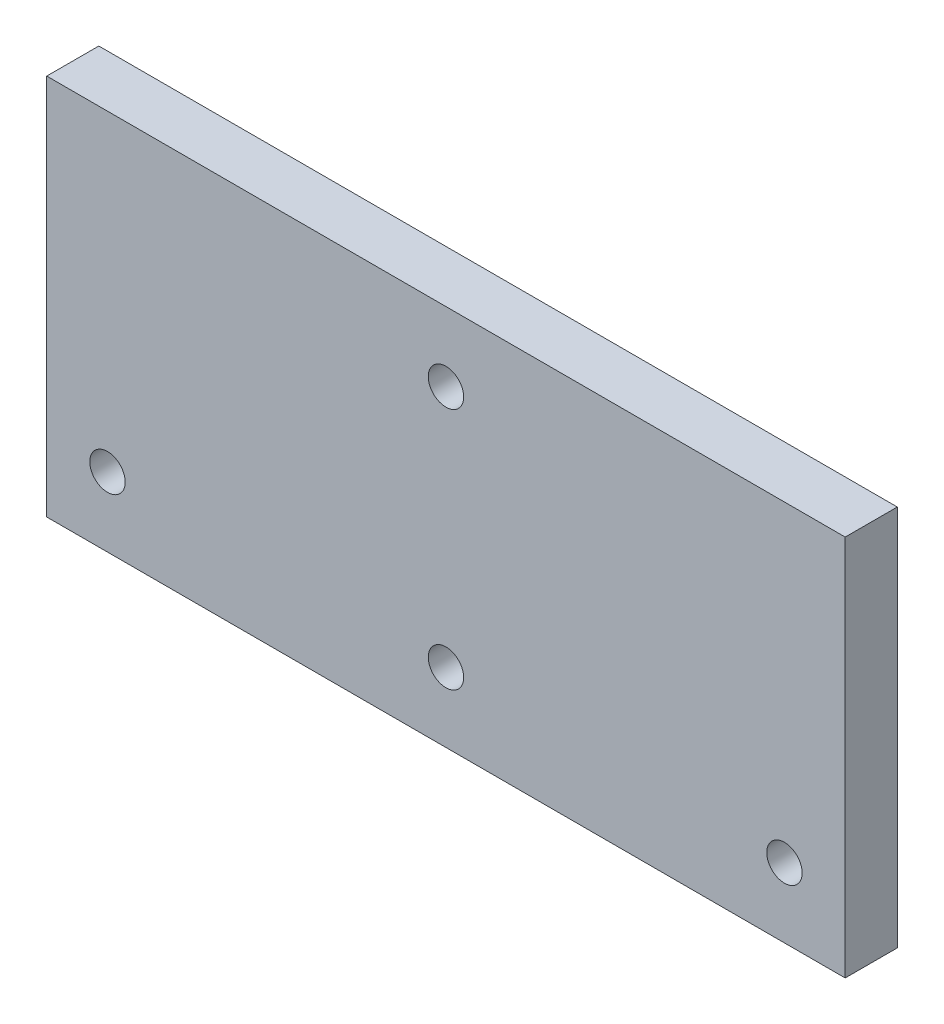
SolidWorks part; units mm, degrees
material "1023 碳钢板 (SS)"
ref_plane "Front Plane" through (0, 0, 0) normal (0, 0, 1) x (1, 0, 0)
ref_plane "Top Plane" through (0, 0, 0) normal (0, 1, 0) x (1, 0, 0)
ref_plane "Right Plane" through (0, 0, 0) normal (1, 0, 0) x (0, 0, -1)
sketch "Sketch1" plane through (0, 0, 0) normal (0, 0, 1) x (1, 0, 0)
  line L1 (-115, 55) -> (115, 55)
  line L2 (-115, 55) -> (-115, -55)
  line L3 (-115, -55) -> (115, -55)
  line L4 (115, 55) -> (115, -55)
  line L5 (-115, 55) -> (115, -55) construction
  line L6 (-115, -55) -> (115, 55) construction
  point P0 (0, 0)
  dimension "D1" = 230
  dimension "D2" = 110
extrude "Boss-Extrude1" add sketch "Sketch1" along normal blind 15
sketch "Sketch8" plane through (0, 0, 15) normal (0, 0, 1) x (1, 0, 0)
  line L3 (-115, 55) -> (-115, -55) construction
  circle A0 centre (-97.5, 35) radius 4
  circle A1 centre (97.5, 35) radius 4
  circle A2 centre (97.5, -35) radius 4
  circle A3 centre (-97.5, -35) radius 4
  circle A4 centre (0, -35) radius 6.5957
  circle A5 centre (0, 35) radius 7.4162
  dimension "D3" = 195
  dimension "D4" = 17.5
  dimension "D5" = 8
  dimension "D1" = 70
  dimension "D2" = 35
hole_wizard "M12 Tapped Hole2" positions "Sketch9" profile "Sketch10" tap size "M12" standard "ISO"
sketch "Sketch9" plane through (0, 0, 15) normal (0, 0, 1) x (1, 0, 0)
  point P3 (-97.5, -35)
  point P9 (97.5, -35)
  point P13 (0, 35)
  point P15 (0, -35)
sketch "Sketch10" plane through (-97.5, -35, 15) normal (1, 0, 0) x (0, -1, 0)
  line L0 (0, 0) -> (0, 32.3144)
  line L1 (0, 32.3144) -> (5.1, 29.25)
  line L2 (5.1, 29.25) -> (5.1, 0)
  line L5 (5.1, 0) -> (0, 0)
  line L10 (0, 32.3144) -> (-5.1, 29.25) construction
  line L11 (0, -6.35) -> (0, 107.95) construction
  dimension "螺纹孔钻头直径" = 10.2
  dimension "螺纹孔钻头深度" = 29.25
  dimension "导头角度" = 118
cosmetic thread "Hole Thread Line7"
cosmetic thread "Hole Thread Line8"
cosmetic thread "Hole Thread Line9"
cosmetic thread "Hole Thread Line10"
